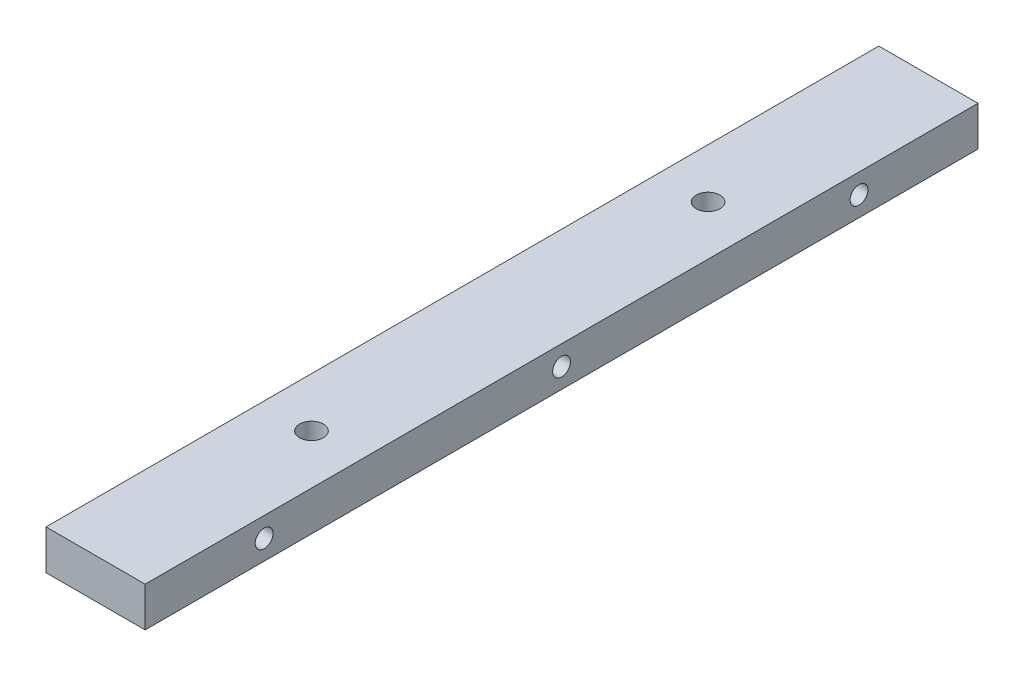
SolidWorks part; units mm, degrees
material "电木（PF）"
ref_plane "前视基准面" through (0, 0, 0) normal (0, 0, 1) x (1, 0, 0)
ref_plane "上视基准面" through (0, 0, 0) normal (0, 1, 0) x (1, 0, 0)
ref_plane "右视基准面" through (0, 0, 0) normal (1, 0, 0) x (0, 0, -1)
sketch "草图1" plane through (0, 0, 0) normal (1, 0, 0) x (0, 0, -1)
  line L1 (-105, 5) -> (105, 5)
  line L2 (-105, 5) -> (-105, -5)
  line L3 (-105, -5) -> (105, -5)
  line L4 (105, 5) -> (105, -5)
  line L5 (-105, 5) -> (105, -5) construction
  line L6 (-105, -5) -> (105, 5) construction
  point P0 (0, 0)
  dimension "D1" = 210
  dimension "D2" = 10
extrude "凸台-拉伸1" add sketch "草图1" along normal mid plane 25
hole_wizard "打孔尺寸(%根据)开槽圆柱头螺钉的类型1" positions "草图2" profile "草图4" counterbore size "M4" standard "GB" end condition through all
sketch "草图2" plane through (-12.5, 0, 0) normal (-1, 0, 0) x (0, 0, 1)
  line L0 (0, 0) -> (0, -38.8742) construction
  point P0 (0, 0)
  point P3 (-75, 0)
  point P9 (75, 0)
  dimension "D1" = 150
sketch "草图4" plane through (-12.5, 0, 0) normal (0, 1, 0) x (0, 0, 1)
  line L0 (0, 0) -> (0, 25)
  line L1 (0, 25) -> (2.25, 25)
  line L3 (2.25, 25) -> (2.25, 5)
  line L4 (2.25, 5) -> (4, 5)
  line L5 (4, 5) -> (4, 0)
  line L7 (4, 0) -> (0, 0)
  line L11 (0, -6.35) -> (0, 107.95) construction
  dimension "通孔孔直径" = 4.5
  dimension "通孔孔深度" = 25
  dimension "柱形沉头孔直径" = 8
  dimension "柱形沉头孔深度" = 5
sketch "草图5" plane through (0, -5, 0) normal (0, -1, 0) x (1, 0, 0)
  line L0 (0, 0) -> (38.2707, 0) construction
  circle A0 centre (0, 50.5635) radius 3
  circle A1 centre (0, -49.4365) radius 3
  dimension "D2" = 6
  dimension "D1" = 100
extrude "切除-拉伸1" cut sketch "草图5" against normal blind 29
